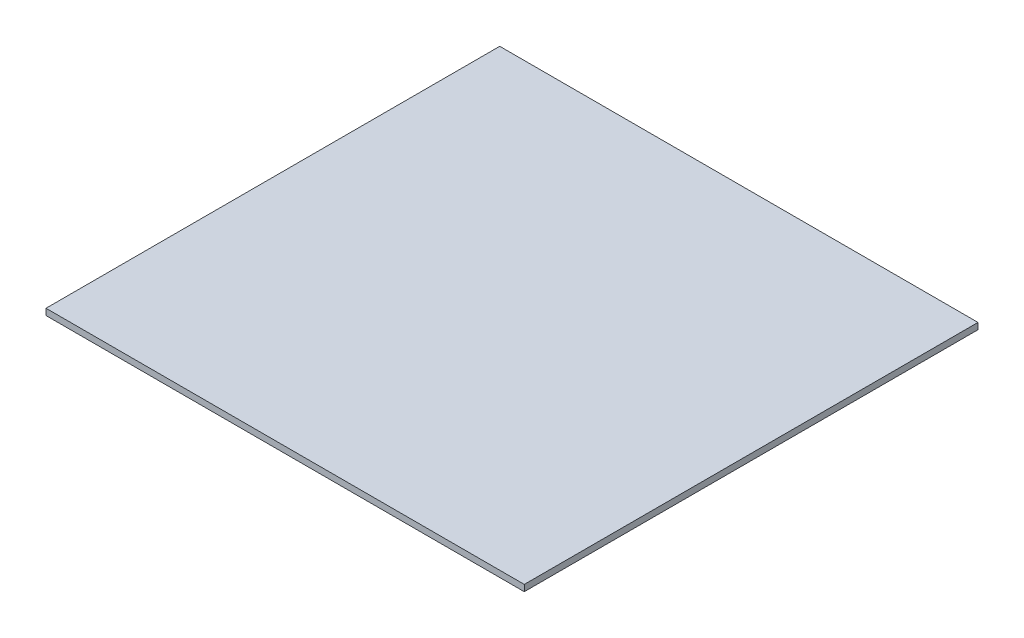
from build123d import *

# Parameters (mm, degrees)
SKETCH_1_W      = 1130
SKETCH_1_H      = 1072
EXTRUDE_1_DEPTH = 15


with BuildPart() as part:
    # 草图1 → 凸台-拉伸1 (new body)
    with BuildSketch(Plane(origin=(0, 0, 0), x_dir=(1, 0, 0), z_dir=(0, 1, 0))):
        Rectangle(SKETCH_1_W, SKETCH_1_H)
    extrude(amount=EXTRUDE_1_DEPTH)


solid = part.part
